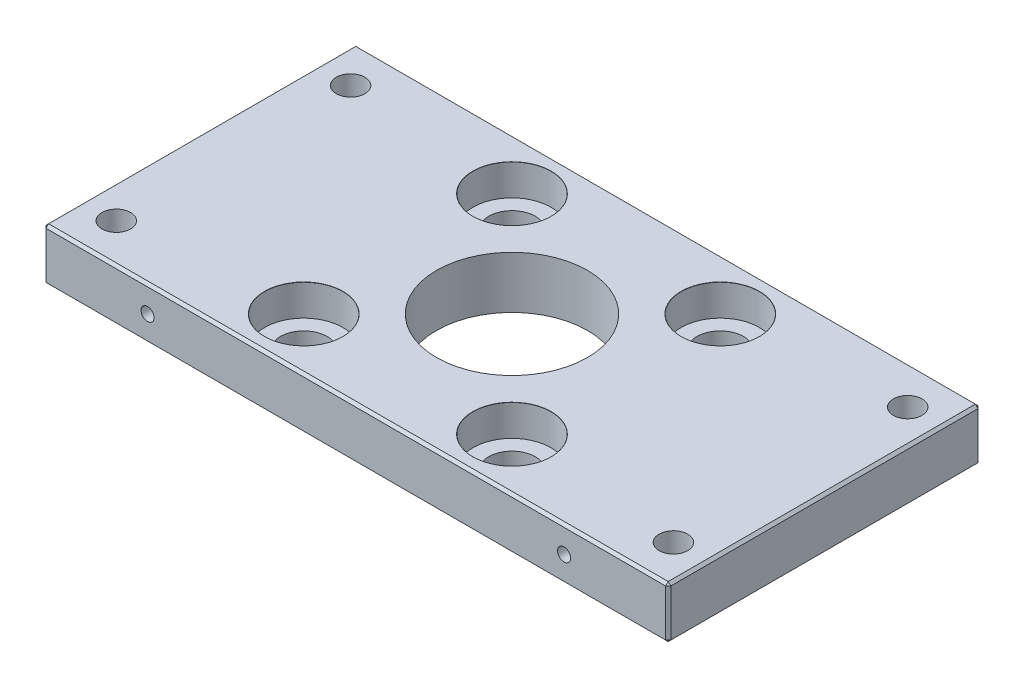
from build123d import *

# Parameters (mm, degrees)
SKETCH1_W                                    = 120
SKETCH1_H                                    = 60
BOSS_EXTRUDE1_DEPTH                          = 10
SKETCH2_R                                    = 14.5
CUT_EXTRUDE1_DEPTH                           = 10
CBORE_FOR_M8_SLOTTED_CHEESE_HEAD_SCR_2_COUNT = 2
CBORE_FOR_M8_SLOTTED_CHEESE_HEAD_SCR_2_PITCH = 56.568542495
CBORE_FOR_M8_SLOTTED_CHEESE_HEAD_SCR_3_COUNT = 2
CBORE_FOR_M8_SLOTTED_CHEESE_HEAD_SCR_3_PITCH = 40
CBORE_FOR_M8_SLOTTED_CHEESE_HEAD_SCR_4_COUNT = 2
CBORE_FOR_M8_SLOTTED_CHEESE_HEAD_SCR_4_PITCH = 40
CBORE_FOR_M5_SLOTTED_CHEESE_HEAD_SCR_2_COUNT = 2
CBORE_FOR_M5_SLOTTED_CHEESE_HEAD_SCR_2_PITCH = 45
CBORE_FOR_M5_SLOTTED_CHEESE_HEAD_SCR_3_COUNT = 2
CBORE_FOR_M5_SLOTTED_CHEESE_HEAD_SCR_3_PITCH = 107
CBORE_FOR_M5_SLOTTED_CHEESE_HEAD_SCR_4_COUNT = 2
CBORE_FOR_M5_SLOTTED_CHEESE_HEAD_SCR_4_PITCH = 116.077560278
M3_TAPPED_HOLE1_D                            = 2.5
M3_TAPPED_HOLE1_DEPTH                        = 12
M3_TAPPED_HOLE1_TIP                          = 0.751075774
CHAMFER1_SIZE                                = 0.5


with BuildPart() as part:
    # Sketch1 → Boss-Extrude1 (new body)
    with BuildSketch(Plane(origin=(0, 0, 0), x_dir=(1, 0, 0), z_dir=(0, 1, 0))):
        with Locations((60, 30)):
            Rectangle(SKETCH1_W, SKETCH1_H)
    extrude(amount=BOSS_EXTRUDE1_DEPTH)

    # Sketch2 → Cut-Extrude1 (cut)
    with BuildSketch(Plane(origin=(0, 10, 0), x_dir=(1, 0, 0), z_dir=(0, 1, 0))):
        with Locations(Location((60, 30, 0), (0, 0, 270))):
            Circle(SKETCH2_R)
    extrude(amount=-CUT_EXTRUDE1_DEPTH, mode=Mode.SUBTRACT)

    # Sketch5 → CBORE for M8 Slotted cheese head screws1 (revolve, cut)
    with BuildSketch(Plane(origin=(80, 10, -10), x_dir=(0, 0, 1), z_dir=(1, 0, 0))):
        Polygon((0, 0), (0, 10), (4.5, 10), (4.5, 6), (7.5, 6), (7.5, 0.025), (7.525, 0), align=None)
    cbore_for_m8_slotted_cheese_head_screws1 = revolve(axis=Axis((80, 16.35, -10), (0, -1, 0)), mode=Mode.SUBTRACT)

    # CBORE for M8 Slotted cheese head scr 2: CBORE for M8 Slotted cheese head screws1 ×2
    with Locations(*[Vector(-0.7071067811865476, 0, -0.7071067811865476) * (i * CBORE_FOR_M8_SLOTTED_CHEESE_HEAD_SCR_2_PITCH) for i in range(1, CBORE_FOR_M8_SLOTTED_CHEESE_HEAD_SCR_2_COUNT)]):
        add(cbore_for_m8_slotted_cheese_head_screws1, mode=Mode.SUBTRACT)

    # CBORE for M8 Slotted cheese head scr 3: CBORE for M8 Slotted cheese head screws1 ×2
    with Locations(*[(0, 0, -i * CBORE_FOR_M8_SLOTTED_CHEESE_HEAD_SCR_3_PITCH) for i in range(1, CBORE_FOR_M8_SLOTTED_CHEESE_HEAD_SCR_3_COUNT)]):
        add(cbore_for_m8_slotted_cheese_head_screws1, mode=Mode.SUBTRACT)

    # CBORE for M8 Slotted cheese head scr 4: CBORE for M8 Slotted cheese head screws1 ×2
    with Locations(*[(-i * CBORE_FOR_M8_SLOTTED_CHEESE_HEAD_SCR_4_PITCH, 0, 0) for i in range(1, CBORE_FOR_M8_SLOTTED_CHEESE_HEAD_SCR_4_COUNT)]):
        add(cbore_for_m8_slotted_cheese_head_screws1, mode=Mode.SUBTRACT)

    # Sketch7 → CBORE for M5 Slotted cheese head screws1 (revolve, cut)
    with BuildSketch(Plane(origin=(6.5, 0, -7.5), x_dir=(0, 0, -1), z_dir=(1, 0, 0))):
        Polygon((0, 0), (0, 10), (2.75, 10), (2.75, 5.7), (5, 5.7), (5, 0.025), (5.025, 0), align=None)
    cbore_for_m5_slotted_cheese_head_screws1 = revolve(axis=Axis((6.5, -6.35, -7.5), (0, 1, 0)), mode=Mode.SUBTRACT)

    # CBORE for M5 Slotted cheese head scr 2: CBORE for M5 Slotted cheese head screws1 ×2
    with Locations(*[(0, 0, -i * CBORE_FOR_M5_SLOTTED_CHEESE_HEAD_SCR_2_PITCH) for i in range(1, CBORE_FOR_M5_SLOTTED_CHEESE_HEAD_SCR_2_COUNT)]):
        add(cbore_for_m5_slotted_cheese_head_screws1, mode=Mode.SUBTRACT)

    # CBORE for M5 Slotted cheese head scr 3: CBORE for M5 Slotted cheese head screws1 ×2
    with Locations(*[(i * CBORE_FOR_M5_SLOTTED_CHEESE_HEAD_SCR_3_PITCH, 0, 0) for i in range(1, CBORE_FOR_M5_SLOTTED_CHEESE_HEAD_SCR_3_COUNT)]):
        add(cbore_for_m5_slotted_cheese_head_screws1, mode=Mode.SUBTRACT)

    # CBORE for M5 Slotted cheese head scr 4: CBORE for M5 Slotted cheese head screws1 ×2
    with Locations(*[Vector(0.9217974580453662, 0, -0.3876718281499204) * (i * CBORE_FOR_M5_SLOTTED_CHEESE_HEAD_SCR_4_PITCH) for i in range(1, CBORE_FOR_M5_SLOTTED_CHEESE_HEAD_SCR_4_COUNT)]):
        add(cbore_for_m5_slotted_cheese_head_screws1, mode=Mode.SUBTRACT)

    # M3 Tapped Hole1
    with Locations(Plane.XY):
        with Locations((20, 5), (100, 5)):
            Hole(M3_TAPPED_HOLE1_D / 2, depth=M3_TAPPED_HOLE1_DEPTH)
            with Locations((0, 0, -(M3_TAPPED_HOLE1_DEPTH + M3_TAPPED_HOLE1_TIP / 2))):  # 118° drill point
                Cone(0, M3_TAPPED_HOLE1_D / 2, M3_TAPPED_HOLE1_TIP, mode=Mode.SUBTRACT)

    # Chamfer1
    chamfer1_edges = [part.edges().sort_by_distance(p)[0] for p in [
        (120, 10, -30),
        (60, 10, -60),
        (0, 10, -30),
        (60, 0, -60),
        (120, 0, -30),
        (60, 0, 0),
        (0, 0, -30),
        (0, 5, -60),
        (120, 5, -60),
        (120, 5, 0),
        (0, 5, 0),
        (60, 10, 0),
    ]]
    chamfer(chamfer1_edges, length=CHAMFER1_SIZE)


solid = part.part
